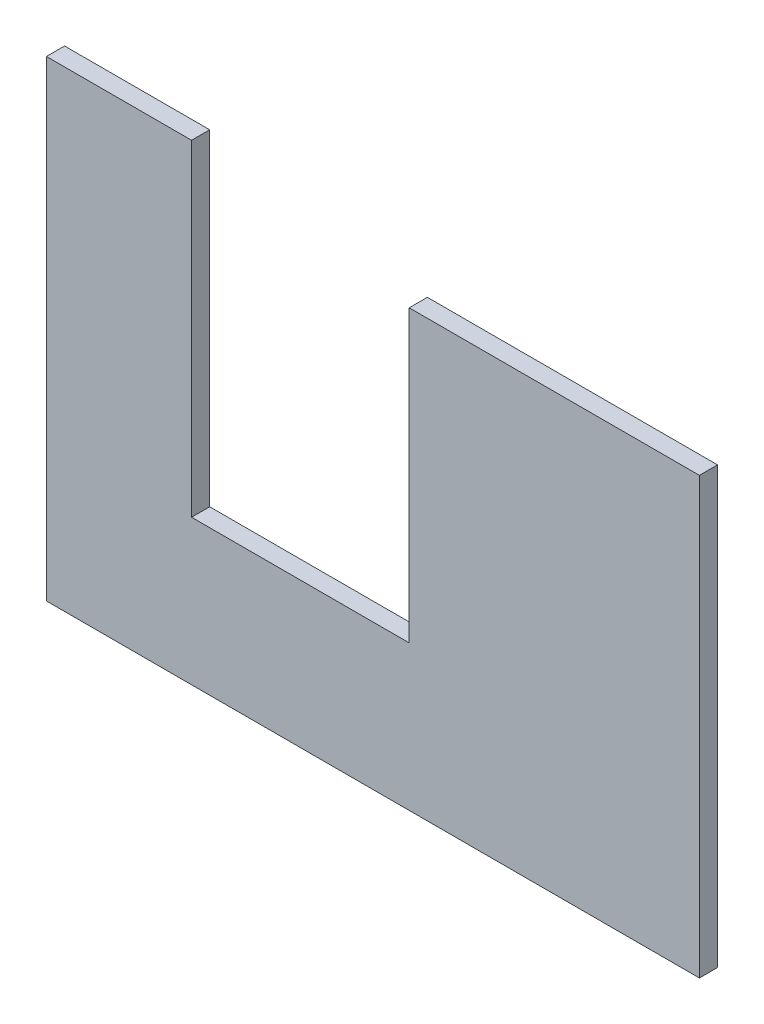
from build123d import *

# Parameters (mm, degrees)
EXTRUDE_1_DEPTH = 5


with BuildPart() as part:
    # 草图1 → 凸台-拉伸1 (new body)
    with BuildSketch(Plane.XY):
        Polygon((0, 0), (0, 130), (40, 130), (40, 40), (100, 40), (100, 120), (180, 120), (180, 0), align=None)
    extrude(amount=EXTRUDE_1_DEPTH)


solid = part.part
